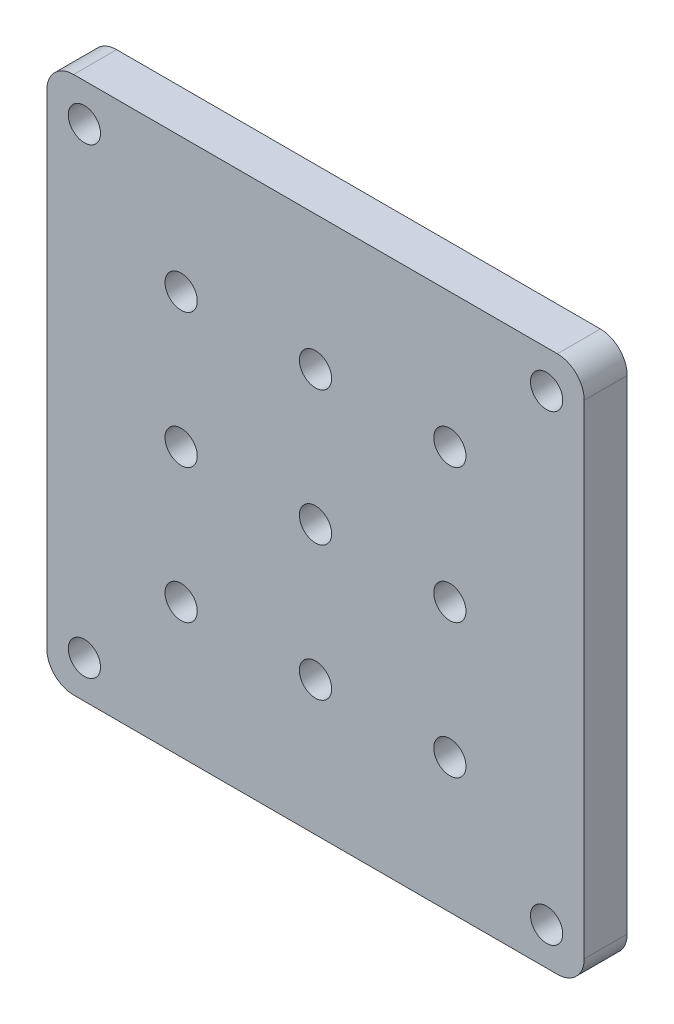
from build123d import *

# Parameters (mm, degrees)
SKETCH1_R           = 3
BOSS_EXTRUDE1_DEPTH = 8


with BuildPart() as part:
    # Sketch1 → Boss-Extrude1 (new body)
    with BuildSketch(Plane.XY):
        with BuildLine():
            Line((-45, 50), (45, 50))
            ThreePointArc((45, 50), (48.535533906, 48.535533906), (50, 45))
            Line((50, 45), (50, -45))
            ThreePointArc((50, -45), (48.535533906, -48.535533906), (45, -50))
            Line((45, -50), (-45, -50))
            ThreePointArc((-45, -50), (-48.535533906, -48.535533906), (-50, -45))
            Line((-50, -45), (-50, 45))
            ThreePointArc((-50, 45), (-48.535533906, 48.535533906), (-45, 50))
        make_face()
        with Locations((-25, 25)):
            Circle(SKETCH1_R, mode=Mode.SUBTRACT)
        with Locations((0, 25)):
            Circle(SKETCH1_R, mode=Mode.SUBTRACT)
        with Locations((25, 25)):
            Circle(SKETCH1_R, mode=Mode.SUBTRACT)
        Circle(SKETCH1_R, mode=Mode.SUBTRACT)
        with Locations((25, 0)):
            Circle(SKETCH1_R, mode=Mode.SUBTRACT)
        with Locations((0, -25)):
            Circle(SKETCH1_R, mode=Mode.SUBTRACT)
        with Locations((25, -25)):
            Circle(SKETCH1_R, mode=Mode.SUBTRACT)
        with Locations((-25, 0)):
            Circle(SKETCH1_R, mode=Mode.SUBTRACT)
        with Locations((-25, -25)):
            Circle(SKETCH1_R, mode=Mode.SUBTRACT)
        with Locations((43, 43)):
            Circle(SKETCH1_R, mode=Mode.SUBTRACT)
        with Locations((43, -43)):
            Circle(SKETCH1_R, mode=Mode.SUBTRACT)
        with Locations((-43, -43)):
            Circle(SKETCH1_R, mode=Mode.SUBTRACT)
        with Locations((-43, 43)):
            Circle(SKETCH1_R, mode=Mode.SUBTRACT)
    extrude(amount=BOSS_EXTRUDE1_DEPTH)


solid = part.part
